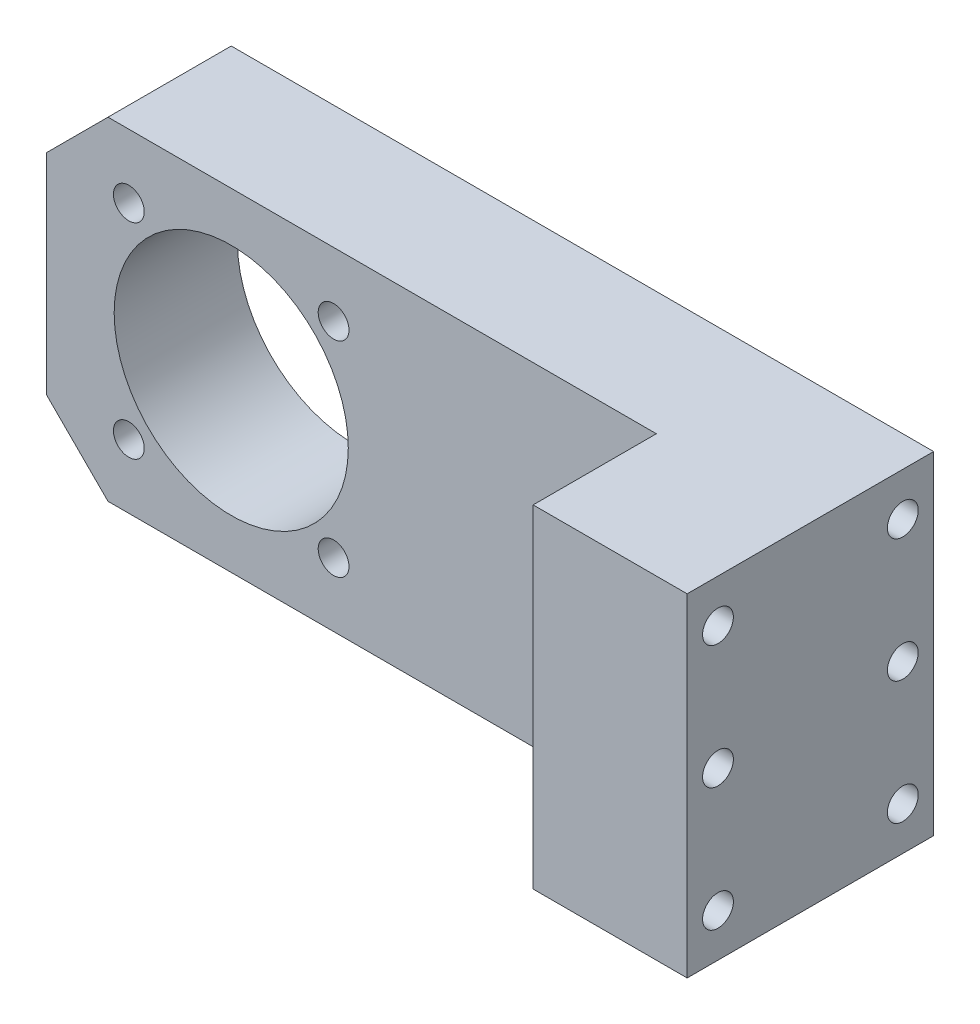
SolidWorks part; units mm, degrees
ref_plane "Front Plane" through (0, 0, 0) normal (0, 0, 1) x (1, 0, 0)
ref_plane "Top Plane" through (0, 0, 0) normal (0, 1, 0) x (1, 0, 0)
ref_plane "Right Plane" through (0, 0, 0) normal (1, 0, 0) x (0, 0, -1)
sketch "Sketch1" plane through (0, 0, 0) normal (0, 0, 1) x (1, 0, 0)
  line L1 (0, 0) -> (124, 0)
  line L2 (0, 0) -> (0, 54)
  line L3 (0, 54) -> (124, 54)
  line L4 (124, 0) -> (124, 54)
  dimension "D1" = 124
  dimension "D2" = 54
extrude "Boss-Extrude1" add sketch "Sketch1" along normal blind 20
chamfer "Chamfer1" distance 10 angle 45 2 edges at (0, 54, 10) (0, 0, 10)
sketch "Sketch2" plane through (0, 0, 20) normal (0, 0, 1) x (1, 0, 0)
  line L0 (10, 0) -> (124, 0) construction
  line L2 (0, 44) -> (0, 10) construction
  circle A0 centre (30, 27) radius 19
  dimension "D1" = 38
  dimension "D2" = 27
  dimension "D3" = 30
extrude "Cut-Extrude1" cut sketch "Sketch2" against normal blind 20
hole_wizard "M6 Tapped Hole1" positions "Sketch6" profile "Sketch5" tap size "M6" standard "GB" end condition through all
sketch "Sketch6" plane through (0, 0, 20) normal (0, 0, 1) x (1, 0, 0)
  line L0 (30, 27) -> (49, 27) construction
  line L2 (30, 27) -> (46.617, 43.617) construction
  circle A0 centre (30, 27) radius 19 construction
  point P1 (46.617, 43.617)
  dimension "D1" = 45
  dimension "D2" = 23.5
cosmetic thread "Cosmetic Thread1" parameters "D2"=6
sketch "Sketch5" plane through (46.617, 43.617, 20) normal (1, 0, 0) x (0, -1, 0)
  line L0 (0, 0) -> (0, 20)
  line L1 (0, 20) -> (2.5, 20)
  line L2 (2.5, 20) -> (2.5, 0)
  line L5 (2.5, 0) -> (0, 0)
  line L11 (0, -6.35) -> (0, 107.95) construction
  dimension "通孔螺纹孔钻头直径" = 5
  dimension "通孔螺纹孔钻头深度" = 20
pattern_circular "CirPattern1" count 4 over 360 about axis through (30, 27, 0) along (0, 0, 1) of "M6 Tapped Hole1"
sketch "Sketch7" plane through (0, 0, 20) normal (0, 0, 1) x (1, 0, 0)
  line L0 (124, 54) -> (10, 54) construction
  line L1 (124, 0) -> (99, 0)
  line L2 (124, 0) -> (124, 54)
  line L3 (124, 54) -> (99, 54)
  line L4 (99, 0) -> (99, 54)
  dimension "D1" = 25
extrude "Boss-Extrude2" add sketch "Sketch7" along normal blind 20
hole_wizard "M6 Tapped Hole2" positions "Sketch9" profile "Sketch8" tap size "M6" standard "Gb"
sketch "Sketch9" plane through (124, 0, 0) normal (1, 0, 0) x (0, 0, -1)
  line L0 (-40, 0) -> (-40, 54) construction
  line L1 (-40, 0) -> (0, 0) construction
  line L2 (-40, 27) -> (5.1565, 27) construction
  point P1 (-35, 47)
  point P3 (-5, 47)
  point P5 (-35, 7)
  point P7 (-5, 7)
  point P22 (-35, 27)
  point P24 (-5, 27)
  dimension "D1" = 40
  dimension "D2" = 30
  dimension "D3" = 5
  dimension "D4" = 7
sketch "Sketch8" plane through (124, 47, 35) normal (0, 1, 0) x (0, 0, -1)
  line L0 (0, 0) -> (0, 16.5022)
  line L1 (0, 16.5022) -> (2.5, 15)
  line L2 (2.5, 15) -> (2.5, 0)
  line L5 (2.5, 0) -> (0, 0)
  line L10 (0, 16.5022) -> (-2.5, 15) construction
  line L11 (0, -6.35) -> (0, 107.95) construction
  dimension "螺纹孔钻头直径" = 5
  dimension "螺纹孔钻头深度" = 15
  dimension "导头角度" = 118
cosmetic thread "Cosmetic Thread2"
cosmetic thread "Cosmetic Thread3"
cosmetic thread "Cosmetic Thread4"
cosmetic thread "Cosmetic Thread5"
cosmetic thread "Cosmetic Thread6"
cosmetic thread "Cosmetic Thread7"
